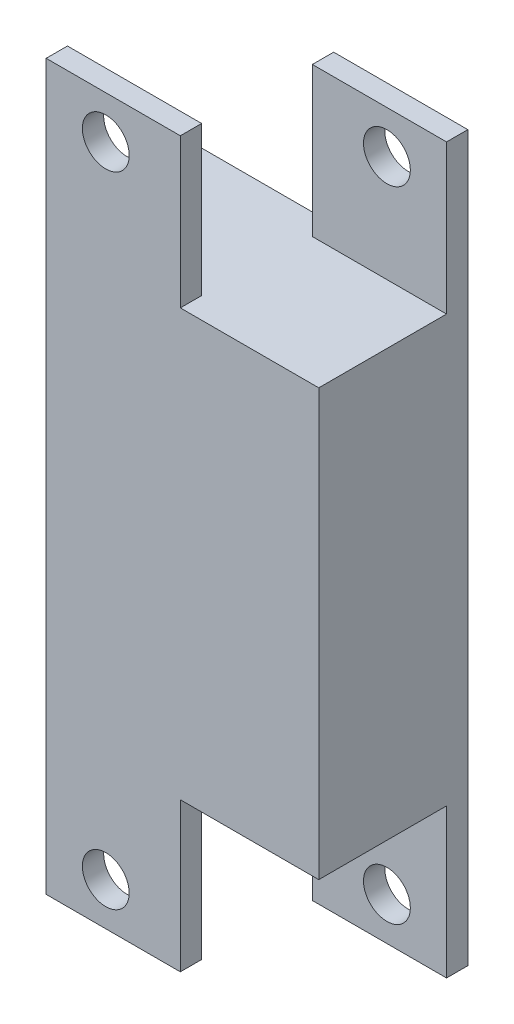
from build123d import *

# Parameters (mm, degrees)
SKETCH_1_W               = 64
SKETCH_1_H               = 170
EXTRUDE_1_DEPTH          = 35
SKETCH_3_W               = 32.5
SKETCH_3_H               = 35
CUT_EXTRUDE_1_DEPTH      = 30
SKETCH_4_W               = 32.5
SKETCH_4_H               = 35
CUT_EXTRUDE_2_DEPTH      = 30
CUT_EXTRUDE_3_DEPTH      = 98.334474879
CUT_EXTRUDE_3_DEPTH_BACK = 98.334474879
SKETCH_5_R               = 5.5


with BuildPart() as part:
    # 草图1 → 凸台-拉伸1 (new body)
    with BuildSketch(Plane.XY):
        Rectangle(SKETCH_1_W, SKETCH_1_H)
    extrude(amount=EXTRUDE_1_DEPTH)

    # 草图3 → 切除-拉伸1 (cut)
    with BuildSketch(Plane.XY.offset(35)):
        with Locations((15.75, 67.5)):
            Rectangle(SKETCH_3_W, SKETCH_3_H)
        with Locations((15.75, -67.5)):
            Rectangle(SKETCH_3_W, SKETCH_3_H)
    extrude(amount=-CUT_EXTRUDE_1_DEPTH, mode=Mode.SUBTRACT)

    # 草图4 → 切除-拉伸2 (cut)
    with BuildSketch(Plane(origin=(0, 0, 0), x_dir=(-1, 0, 0), z_dir=(0, 0, -1))):
        with Locations((15.75, 67.5)):
            Rectangle(SKETCH_4_W, SKETCH_4_H)
        with Locations((15.75, -67.5)):
            Rectangle(SKETCH_4_W, SKETCH_4_H)
    extrude(amount=-CUT_EXTRUDE_2_DEPTH, mode=Mode.SUBTRACT)

    # 草图5 → 切除-拉伸3 (cut, two sides: drawn at the far end of the back side and taken through both)
    with BuildSketch(Plane.XY.offset(35).offset(-CUT_EXTRUDE_3_DEPTH_BACK)):
        with Locations((-18, 75)):
            Circle(SKETCH_5_R)
        with Locations((18, 75)):
            Circle(SKETCH_5_R)
        with Locations((18, -75)):
            Circle(SKETCH_5_R)
        with Locations((-18, -75)):
            Circle(SKETCH_5_R)
    extrude(amount=CUT_EXTRUDE_3_DEPTH + CUT_EXTRUDE_3_DEPTH_BACK, mode=Mode.SUBTRACT)


solid = part.part
